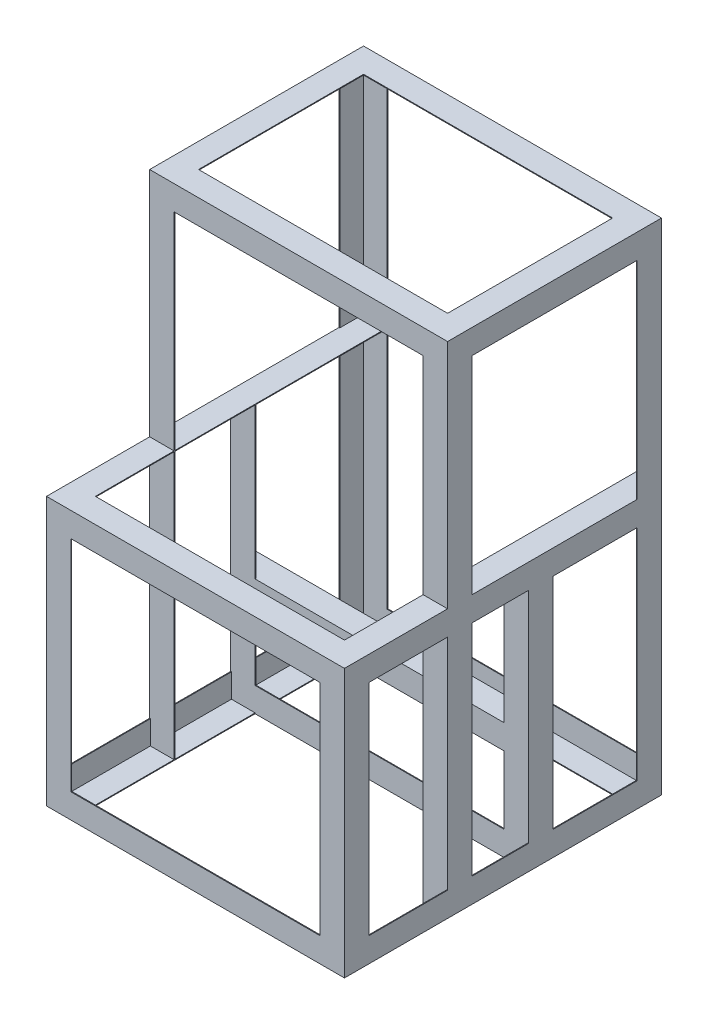
SolidWorks part; units mm, degrees
ref_plane "Front" through (0, 0, 0) normal (0, 0, 1) x (1, 0, 0)
ref_plane "Top" through (0, 0, 0) normal (0, 1, 0) x (1, 0, 0)
ref_plane "Right" through (0, 0, 0) normal (1, 0, 0) x (0, 0, -1)
sketch "Sketch1" plane through (0, 0, 0) normal (0, 1, 0) x (1, 0, 0)
  line L0 (0, 0) -> (0, 64)
  line L1 (0, 64) -> (64, 64)
  line L2 (64, 64) -> (64, 62)
  line L3 (64, 62) -> (2, 62)
  line L4 (2, 62) -> (2, 0)
  line L5 (2, 0) -> (0, 0)
  dimension "D1" = 64
  dimension "D2" = 64
  dimension "D3" = 2
  dimension "D4" = 2
extrude "Boss-Extrude1" add sketch "Sketch1" along normal blind 1308
sketch "Sketch2" plane through (0, 0, -62) normal (0, 0, 1) x (1, 0, 0)
  line L0 (64, 0) -> (0, 0)
  line L1 (0, 0) -> (0, 64)
  line L2 (0, 1308) -> (0, 0) construction
  line L3 (0, 64) -> (2, 64)
  line L4 (2, 1308) -> (2, 0) construction
  line L5 (2, 64) -> (2, 2)
  line L6 (2, 2) -> (64, 2)
  line L7 (64, 1308) -> (64, 0) construction
  line L8 (64, 2) -> (64, 0)
  dimension "D1" = 2
  dimension "D2" = 64
extrude "Boss-Extrude2" add sketch "Sketch2" along normal blind 828
sketch "Sketch3" plane through (0, 2, 0) normal (0, 1, 0) x (1, 0, 0)
  line L0 (64, -766) -> (0, -766)
  line L1 (0, -766) -> (0, -702)
  line L2 (0, -766) -> (0, 0) construction
  line L3 (0, -702) -> (2, -702)
  line L4 (2, -766) -> (2, 0) construction
  line L5 (2, -702) -> (2, -764)
  line L6 (2, -766) -> (2, 62) construction
  line L7 (2, -764) -> (64, -764)
  line L8 (64, -766) -> (64, 62) construction
  line L9 (64, -764) -> (64, -766)
  dimension "D1" = 64
  dimension "D2" = 2
extrude "Boss-Extrude3" add sketch "Sketch3" along normal blind 700
sketch "Sketch4" plane through (0, 0, 764) normal (0, 0, -1) x (-1, 0, 0)
  line L0 (-64, 702) -> (0, 702)
  line L1 (0, 702) -> (0, 638)
  line L2 (0, 638) -> (-2, 638)
  line L4 (-2, 702) -> (-2, 2) construction
  line L5 (-2, 638) -> (-2, 700)
  line L6 (-2, 702) -> (-2, 64) construction
  line L7 (-2, 700) -> (-64, 700)
  line L8 (-64, 702) -> (-64, 2) construction
  line L9 (-64, 702) -> (-64, 700)
  dimension "D1" = 2
  dimension "D2" = 64
extrude "Boss-Extrude4" add sketch "Sketch4" along normal blind 828 contours L7 L9 L0 L1 L2 L5
sketch "Sketch5" plane through (0, 0, -62) normal (0, 0, 1) x (1, 0, 0)
  line L0 (64, 1308) -> (0, 1308)
  line L1 (0, 1308) -> (0, 1244)
  line L2 (0, 1308) -> (0, 702) construction
  line L3 (0, 1244) -> (2, 1244)
  line L4 (2, 1308) -> (2, 702) construction
  line L5 (2, 1244) -> (2, 1306)
  line L6 (2, 1308) -> (2, 702) construction
  line L7 (2, 1306) -> (64, 1306)
  line L8 (64, 1308) -> (64, 702) construction
  line L9 (64, 1306) -> (64, 1308)
  dimension "D1" = 64
  dimension "D2" = 2
extrude "Boss-Extrude5" add sketch "Sketch5" along normal blind 558
sketch "Sketch6" plane through (0, 1306, 0) normal (0, -1, 0) x (1, 0, 0)
  line L0 (64, 496) -> (0, 496)
  line L1 (0, 496) -> (0, 432)
  line L2 (0, -64) -> (0, 496) construction
  line L3 (0, 432) -> (2, 432)
  line L4 (2, 432) -> (2, 494)
  line L5 (2, 494) -> (64, 494)
  line L6 (64, 496) -> (64, -64) construction
  line L7 (64, 494) -> (64, 496)
  dimension "D1" = 2
  dimension "D2" = 64
  dimension "D3" = 2
extrude "Boss-Extrude6" add sketch "Sketch6" along normal up to surface (1304 mm away) up to face at (33, 2, 351)
sketch "Sketch7" plane through (2, 0, 0) normal (1, 0, 0) x (0, 0, -1)
  line L0 (-496, 1308) -> (-432, 1308)
  line L1 (-496, 1308) -> (64, 1308) construction
  line L2 (-432, 1308) -> (-432, 1306)
  line L3 (-432, 1306) -> (-494, 1306)
  line L4 (-494, 1306) -> (-494, 1244)
  line L5 (-494, 1244) -> (-496, 1244)
  line L6 (-496, 702) -> (-496, 1308) construction
  line L7 (-496, 1244) -> (-496, 1308)
  line L8 (64, 1308) -> (0, 1308)
  line L9 (0, 1308) -> (0, 1306)
  line L10 (-494, 1306) -> (62, 1306) construction
  line L11 (0, 1306) -> (62, 1306)
  line L12 (62, 1306) -> (62, 1244)
  line L13 (62, 1306) -> (62, 702) construction
  line L14 (62, 1244) -> (64, 1244)
  line L15 (64, 1308) -> (64, 0) construction
  line L16 (64, 1244) -> (64, 1308)
  line L17 (64, 0) -> (64, 64)
  line L18 (64, 64) -> (62, 64)
  line L19 (62, 700) -> (62, 2) construction
  line L20 (62, 64) -> (62, 2)
  line L21 (62, 2) -> (0, 2)
  line L22 (-494, 2) -> (62, 2) construction
  line L23 (0, 2) -> (0, 0)
  line L24 (0, 0) -> (64, 0)
  line L25 (-766, 0) -> (-766, 64)
  line L26 (-766, 0) -> (-766, 702) construction
  line L27 (-766, 64) -> (-763.7558, 64)
  line L28 (-763.7558, 64) -> (-764, 2)
  line L29 (-764, 2) -> (-702, 2)
  line L30 (-764, 2) -> (-496, 2) construction
  line L31 (-702, 2) -> (-702, 0)
  line L32 (-766, 0) -> (64, 0) construction
  line L33 (-702, 0) -> (-766, 0)
  line L34 (-766, 702) -> (-702, 702)
  line L35 (-766, 702) -> (-496, 702) construction
  line L36 (-702, 702) -> (-702, 700)
  line L37 (-496, 700) -> (-764, 700) construction
  line L38 (-702, 700) -> (-764, 700)
  line L39 (-764, 700) -> (-764, 638)
  line L40 (-764, 700) -> (-764, 2) construction
  line L41 (-764, 638) -> (-766, 638)
  line L42 (-766, 638) -> (-766, 702)
  dimension "D1" = 2
  dimension "D2" = 2
  dimension "D3" = 64
  dimension "D4" = 64
  dimension "D5" = 64
  dimension "D6" = 64
  dimension "D7" = 64
  dimension "D8" = 64
  dimension "D9" = 64
  dimension "D10" = 64
  dimension "D11" = 64
  dimension "D12" = 64
extrude "Boss-Extrude8" add sketch "Sketch7" along normal blind 388
ref_plane "Plane1" through (390, 0, 0) normal (1, 0, 0) x (0, 0, -1)
mirror "Mirror3" about plane through (390, 0, 0) normal (1, 0, 0) of "Boss-Extrude8", "Boss-Extrude6", "Boss-Extrude5", "Boss-Extrude4", "Boss-Extrude3", "Boss-Extrude2", "Boss-Extrude1"
mirror "Mirror4" about plane through (390, 0, 0) normal (1, 0, 0) of "Mirror3"
sketch "Sketch8" plane through (0, 0, 0) normal (0, -1, 0) x (1, 0, 0)
  line L0 (0, 283.8162) -> (64, 283.8162)
  line L1 (0, -64) -> (0, 766) construction
  line L2 (64, 702) -> (64, 0) construction
  line L3 (64, 283.8162) -> (64, 281.8162)
  line L4 (64, 281.8162) -> (2, 281.8162)
  line L5 (2, 281.8162) -> (2, 219.8162)
  line L6 (2, 219.8162) -> (0, 219.8162)
  line L7 (0, 219.8162) -> (0, 283.8162)
  dimension "D1" = 2
  dimension "D2" = 2
  dimension "D3" = 64
extrude "Boss-Extrude9" add sketch "Sketch8" against normal up to surface (700 mm away) up to face at (33, 700, 216)
mirror "Mirror5" about plane through (390, 0, 0) normal (1, 0, 0) of "Boss-Extrude9"
sketch "Sketch9" plane through (0, 0, 0) normal (-1, 0, 0) x (0, 0, 1)
  line L0 (283.8162, 64) -> (283.8162, 0)
  line L1 (-64, 0) -> (766, 0) construction
  line L2 (283.8162, 0) -> (219.8162, 0)
  line L3 (219.8162, 0) -> (219.8162, 2)
  line L4 (219.8162, 2) -> (281.8162, 2)
  line L5 (281.8162, 2) -> (281.8162, 64)
  line L6 (281.8162, 64) -> (283.8162, 64)
  dimension "D1" = 2
  dimension "D2" = 2
  dimension "D3" = 64
extrude "Boss-Extrude10" add sketch "Sketch9" against normal up to surface (778 mm away) up to face at (778, 293.6, 644.3756)
sketch "Sketch10" plane through (0, 0, 0) normal (-1, 0, 0) x (0, 0, 1)
  line L0 (219.8162, 305.5474) -> (283.8162, 305.5474)
  line L1 (219.8162, 638) -> (219.8162, 64) construction
  line L2 (283.8162, 638) -> (283.8162, 64) construction
  line L3 (283.8162, 305.5474) -> (283.8162, 241.5474)
  line L4 (283.8162, 241.5474) -> (281.8162, 241.5474)
  line L5 (281.8162, 241.5474) -> (281.8162, 303.5474)
  line L6 (281.8162, 303.5474) -> (219.8162, 303.5474)
  line L7 (219.8162, 303.5474) -> (219.8162, 305.5474)
  dimension "D1" = 64
  dimension "D2" = 2
  dimension "D3" = 2
extrude "Boss-Extrude11" add sketch "Sketch10" against normal up to surface (778 mm away)
